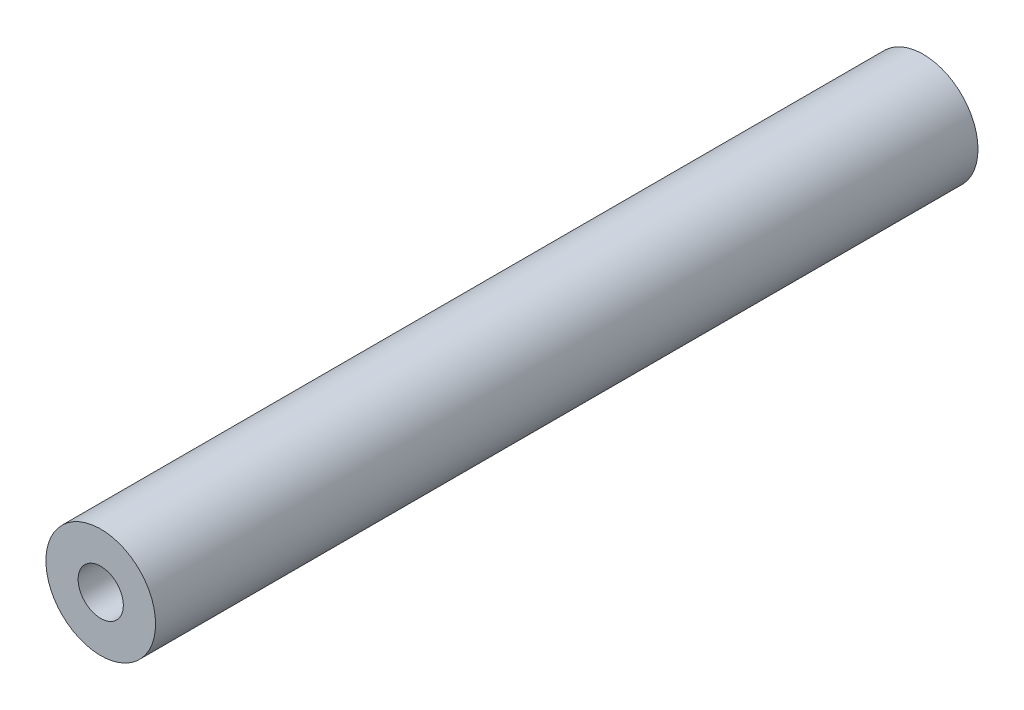
from build123d import *

# Parameters (mm, degrees)
SKETCH_1_R      = 4
SKETCH_1_R_2    = 1.65
EXTRUDE_1_DEPTH = 30


with BuildPart() as part:
    # 草图1 → 凸台-拉伸1 (new, symmetric)
    with BuildSketch(Plane.XY):
        Circle(SKETCH_1_R)
        Circle(SKETCH_1_R_2, mode=Mode.SUBTRACT)
    extrude(amount=EXTRUDE_1_DEPTH, both=True)


solid = part.part
